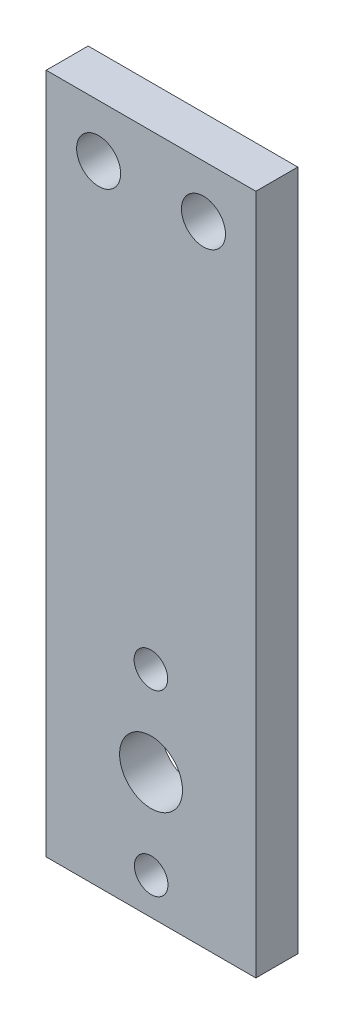
SolidWorks part; units mm, degrees
ref_plane "Front Plane" through (0, 0, 0) normal (0, 0, 1) x (1, 0, 0)
ref_plane "Top Plane" through (0, 0, 0) normal (0, 1, 0) x (1, 0, 0)
ref_plane "Right Plane" through (0, 0, 0) normal (1, 0, 0) x (0, 0, -1)
sketch "Sketch1" plane through (0, 0, 0) normal (0, 0, 1) x (1, 0, 0)
  line L1 (-10, -32.5) -> (10, -32.5)
  line L2 (-10, -32.5) -> (-10, 32.5)
  line L3 (-10, 32.5) -> (10, 32.5)
  line L4 (10, -32.5) -> (10, 32.5)
  line L5 (-10, -32.5) -> (10, 32.5) construction
  line L6 (-10, 32.5) -> (10, -32.5) construction
  circle A0 centre (-5, 27.5) radius 2.1
  circle A1 centre (5, 27.5) radius 2.1
  circle A2 centre (0, -20.5) radius 3
  circle A3 centre (-0.014, -12) radius 1.6
  circle A4 centre (0.014, -29) radius 1.6
  point P0 (0, 0)
  dimension "D2" = 10
  dimension "D3" = 5
  dimension "D5" = 4.2
  dimension "D6" = 4.2
  dimension "D9" = 6
  dimension "D1" = 20
  dimension "D4" = 5
  dimension "D7" = 65
  dimension "D8" = 5
  dimension "D10" = 48
  dimension "D11" = 8.5
  dimension "D12" = 8.5
extrude "Boss-Extrude1" add sketch "Sketch1" along normal blind 4
